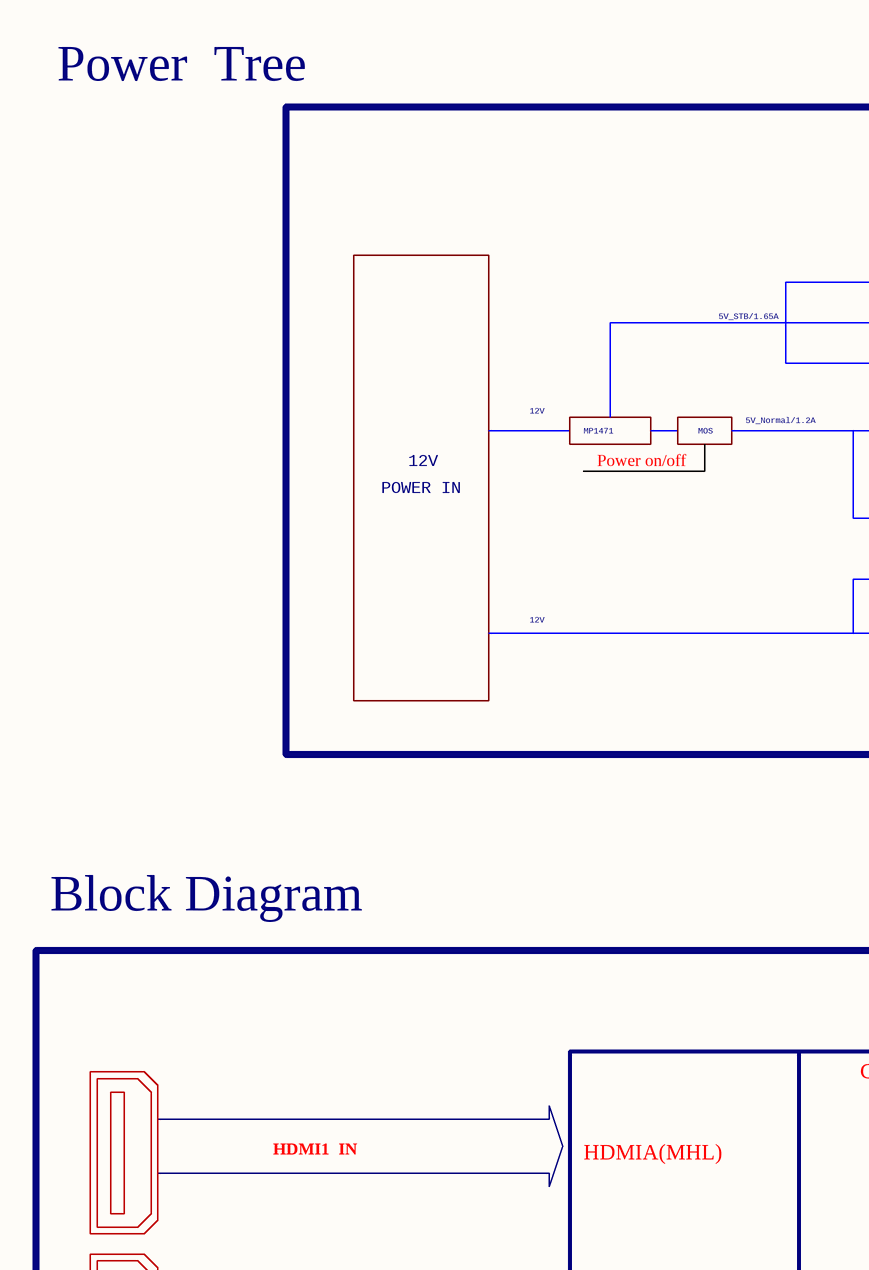
[diagram p0: MISC84277-6.SchDoc, top left]
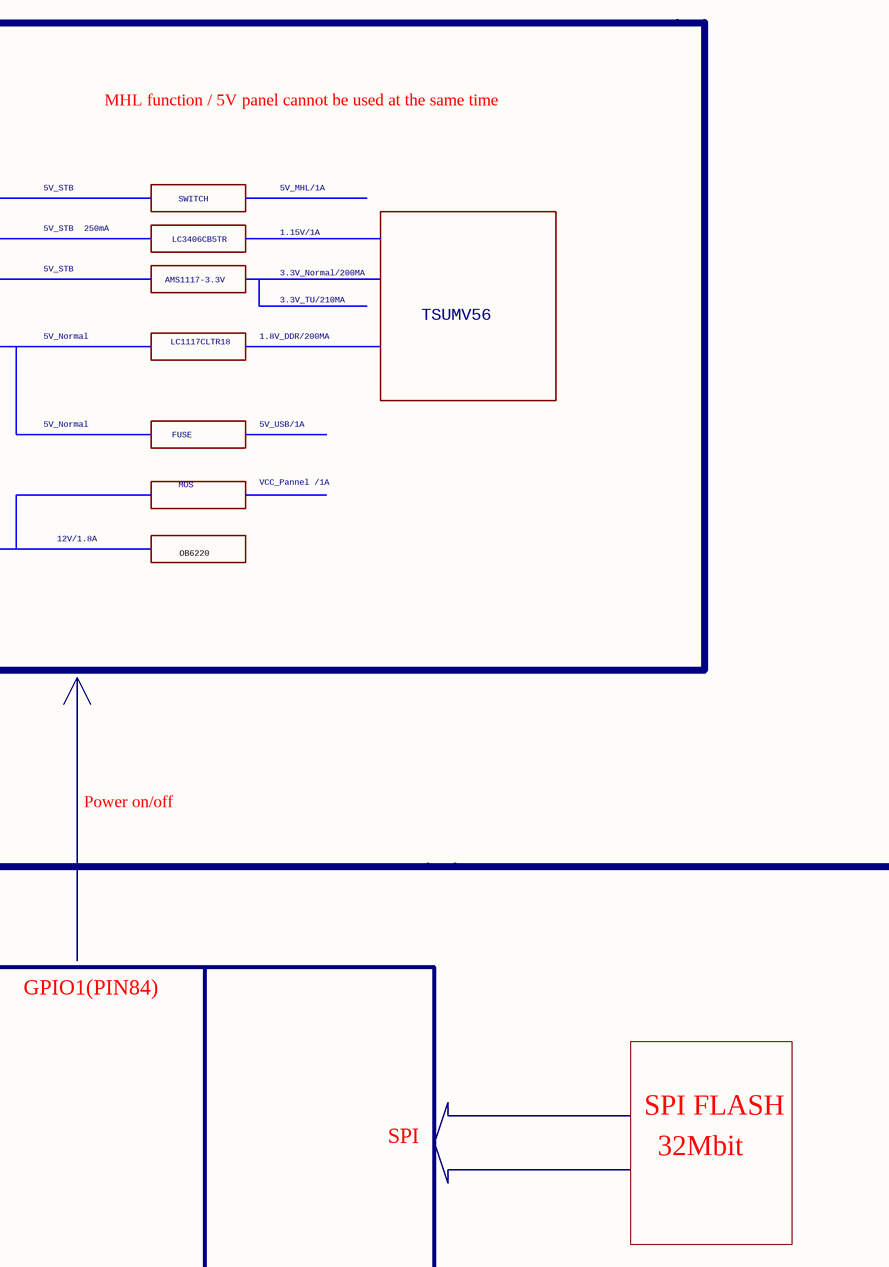
[diagram p1: MISC84277-6.SchDoc, top right]
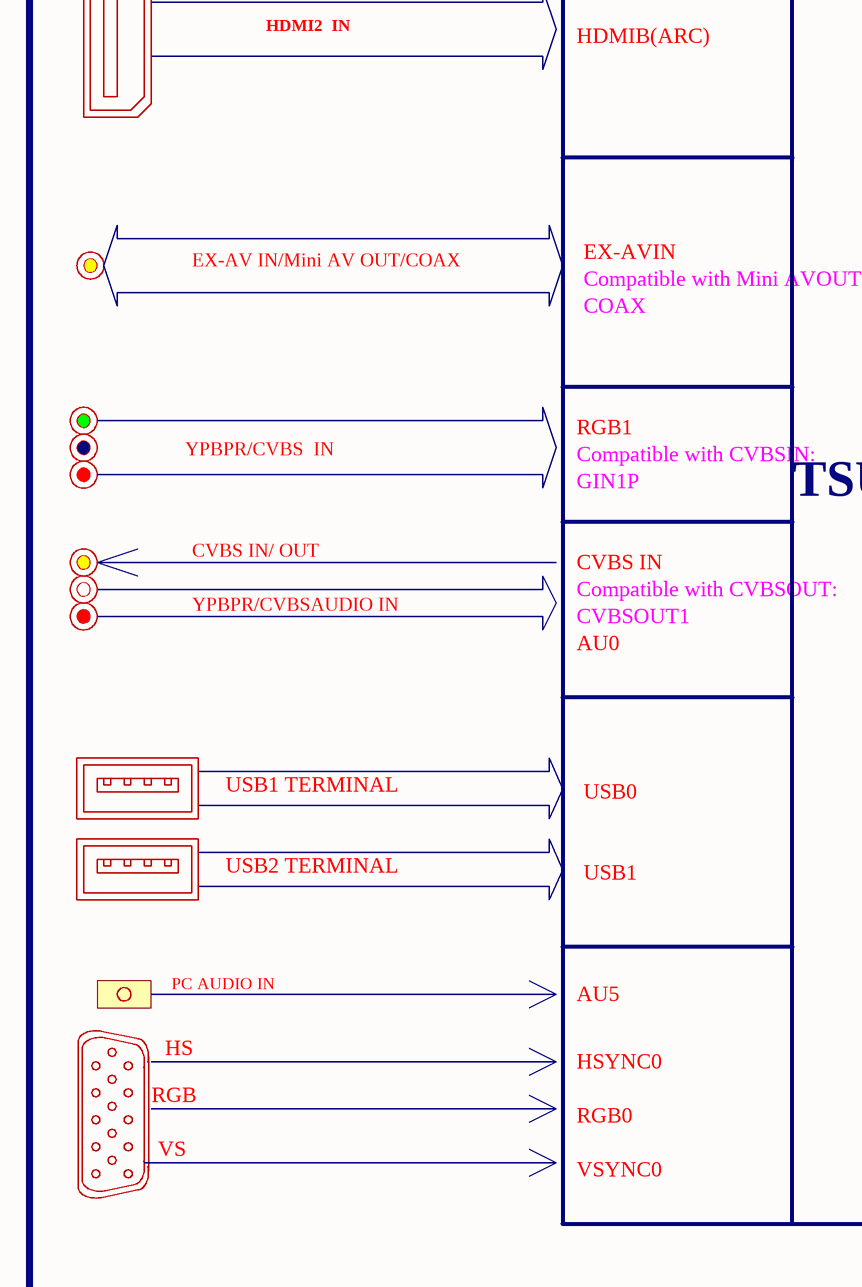
[diagram p2: MISC84277-6.SchDoc, bottom left]
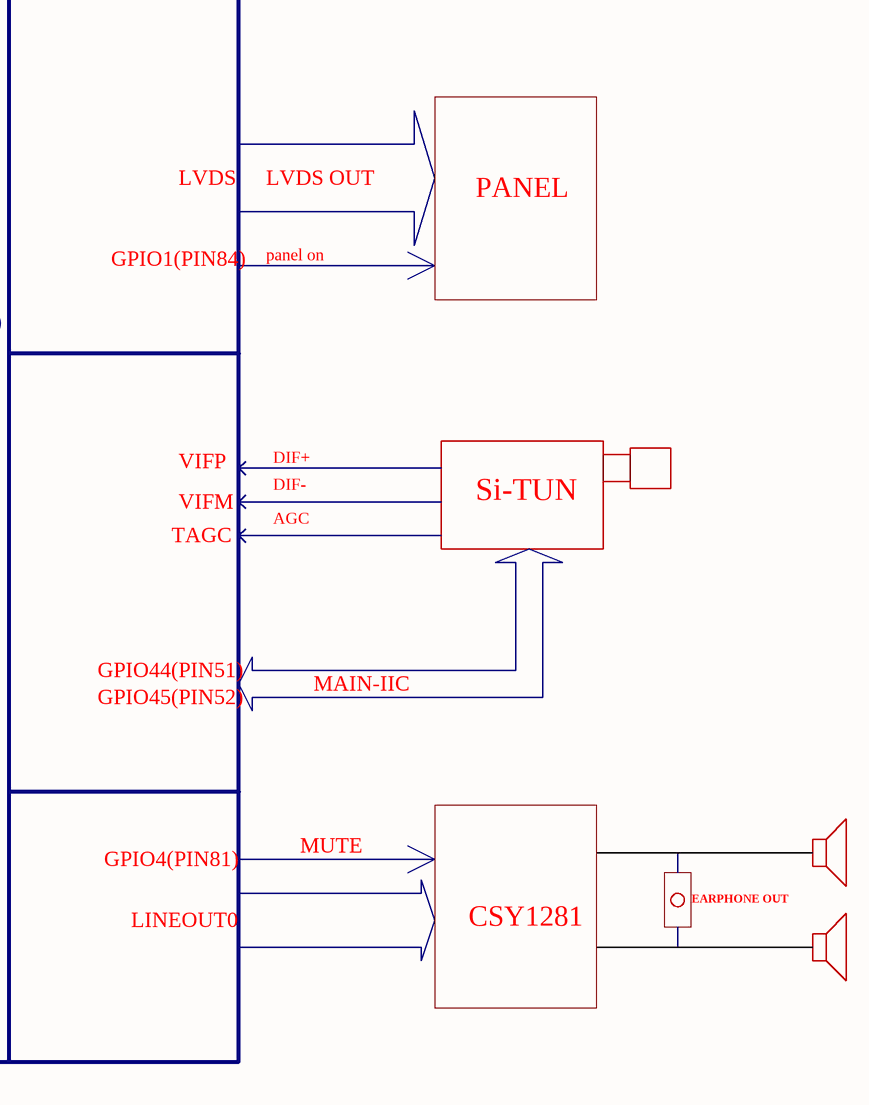
[diagram p3: MISC84277-6.SchDoc, bottom right]
# Altium project MISC84277-14.PrjPCB (part 2 of 10)

## Sheet MISC84277-6.SchDoc
size 401 x 533 mm

### Notes on the sheet
- Power  Tree
- MHL function / 5V panel cannot be used at the same time
- 5V_STB
- SWITCH
- 5V_MHL/1A
- 5V_STB/1.65A
- 250mA
- AMS1117-3.3V
- LC3406CB5TR
- 3.3V_Normal/200MA
- 1.15V/1A
- 12V
- MP1471
- MOS
- 5V_Normal/1.2A
- 5V_Normal
- LC1117CLTR18
- 1.8V_DDR/200MA
- 3.3V_TU/210MA
- TSUMV56
- POWER IN
- Power on/off
- 5V_USB/1A
- FUSE
- VCC_Pannel /1A
- 12V/1.8A
- OB6220
- Block Diagram
- GPIO1(PIN84)
- HDMI1  IN
- HDMIA(MHL)
- SPI
- SPI FLASH
- 32Mbit
- HDMI2  IN
- HDMIB(ARC)
- EX-AV IN/Mini AV OUT/COAX
- EX-AVIN
- Compatible with Mini AVOUT:
- COAX
- LVDS
- LVDS OUT
- PANEL
- panel on
- YPBPR/CVBS  IN
- RGB1
- Compatible with CVBSIN:
- GIN1P
- CVBS IN/ OUT
- YPBPR/CVBSAUDIO IN
- Compatible with CVBSOUT:
- CVBS IN
- CVBSOUT1
- VIFP
- DIF+
- AU0
- VIFM
- DIF-
- AGC
- Si-TUN
- TAGC
- USB1 TERMINAL
- USB0
- USB2 TERMINAL
- USB1
- GPIO44(PIN51)
- GPIO45(PIN52)
- MAIN-IIC
- PC AUDIO IN
- AU5
- GPIO4(PIN81)
- MUTE
- HS
- HSYNC0
- LINEOUT0
- CSY1281
- EARPHONE OUT
- RGB
- VS
- RGB0
- VSYNC0